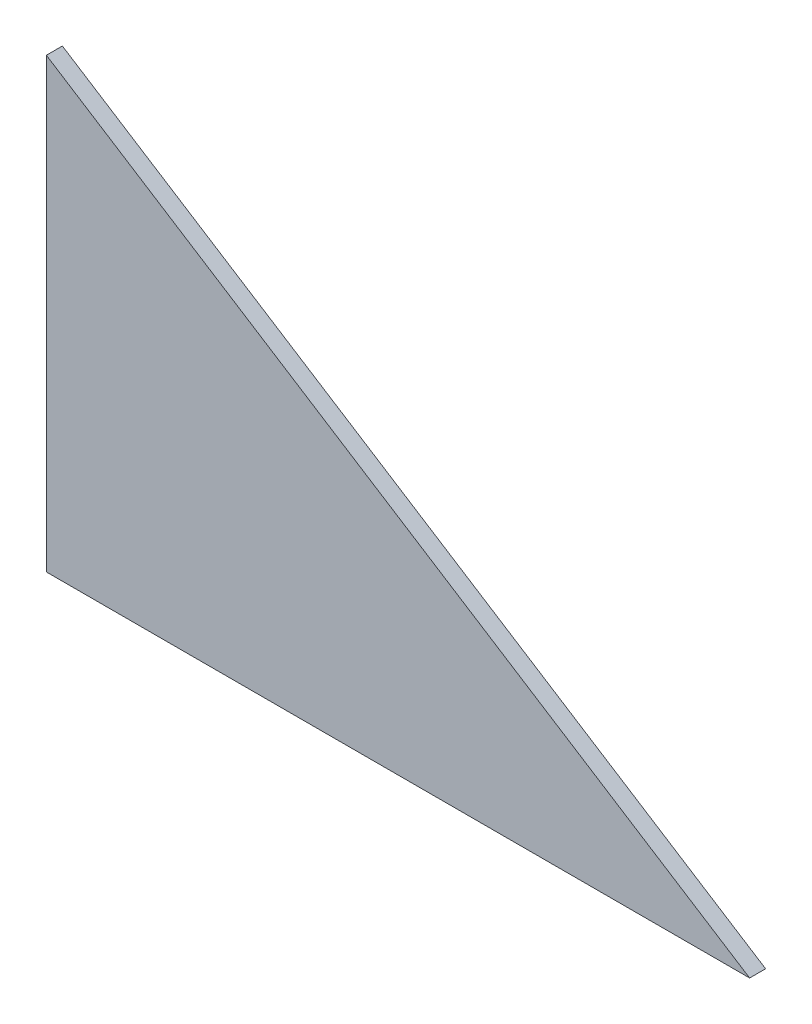
SolidWorks part; units mm, degrees
ref_plane "Front Plane" through (0, 0, 0) normal (0, 0, 1) x (1, 0, 0)
ref_plane "Top Plane" through (0, 0, 0) normal (0, 1, 0) x (1, 0, 0)
ref_plane "Right Plane" through (0, 0, 0) normal (1, 0, 0) x (0, 0, -1)
other "Configuration Table"
sketch "Sketch1" plane through (0, 0, 0) normal (0, 0, 1) x (1, 0, 0)
  line L0 (0, 0) -> (0, 280)
  line L1 (0, 280) -> (440, 0)
  line L2 (440, 0) -> (0, 0)
  dimension "D1" = 280
  dimension "D2" = 440
extrude "Boss-Extrude1" add sketch "Sketch1" along normal blind 10
